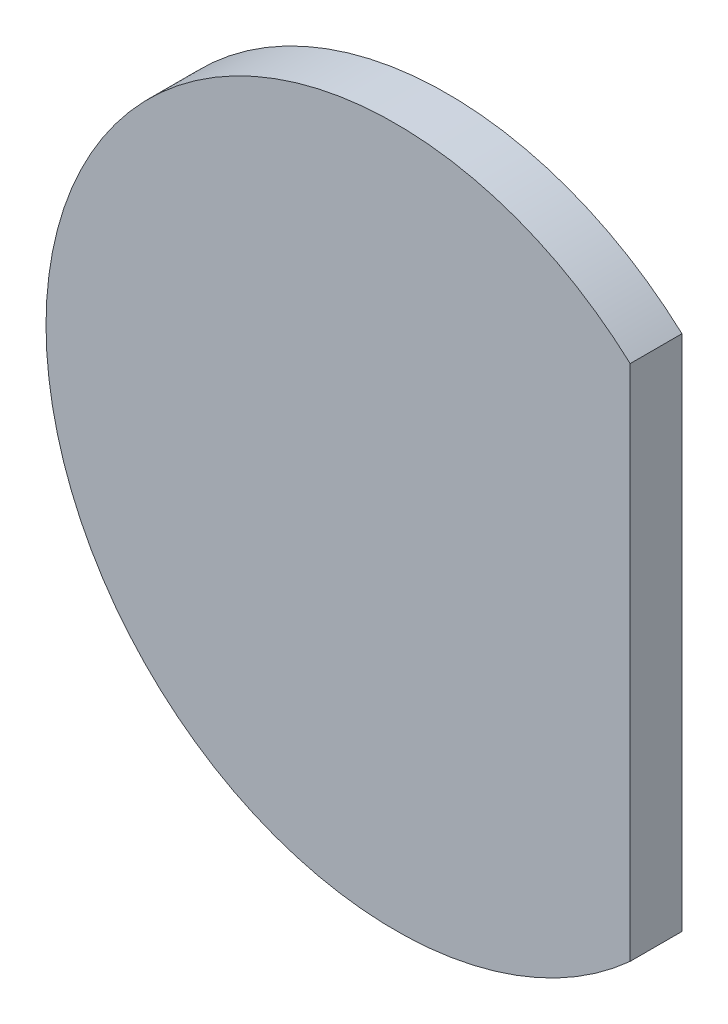
SolidWorks part; units mm, degrees
ref_plane "Front Plane" through (0, 0, 0) normal (0, 0, 1) x (1, 0, 0)
ref_plane "Top Plane" through (0, 0, 0) normal (0, 1, 0) x (1, 0, 0)
ref_plane "Right Plane" through (0, 0, 0) normal (1, 0, 0) x (0, 0, -1)
sketch "Sketch1" plane through (0, 0, 0) normal (0, 0, 1) x (1, 0, 0)
  line L0 (90.69, 100.0016) -> (90.69, -100.0016)
  arc A0 (90.69, 100.0016) -> (90.69, -100.0016) centre (0, 0) ccw
  dimension "D1" = 135
  dimension "D2" = 90.69
extrude "Boss-Extrude1" add sketch "Sketch1" along normal blind 20
sketch "Sketch2" plane through (0, 0, 20) normal (0, 0, 1) x (1, 0, 0)
  line L0 (0, 135) -> (0, -135)
  arc A0 (90.69, 100.0016) -> (90.69, -100.0016) centre (0, 0) ccw construction
sketch "Sketch3" [suppressed] plane through (0, 0, 20) normal (0, 0, 1) x (1, 0, 0)
  line L0 (90.69, 0) -> (-135, 0)
  line L1 (90.69, -100.0016) -> (90.69, 100.0016) construction
  arc A0 (90.69, 100.0016) -> (90.69, -100.0016) centre (0, 0) ccw construction
